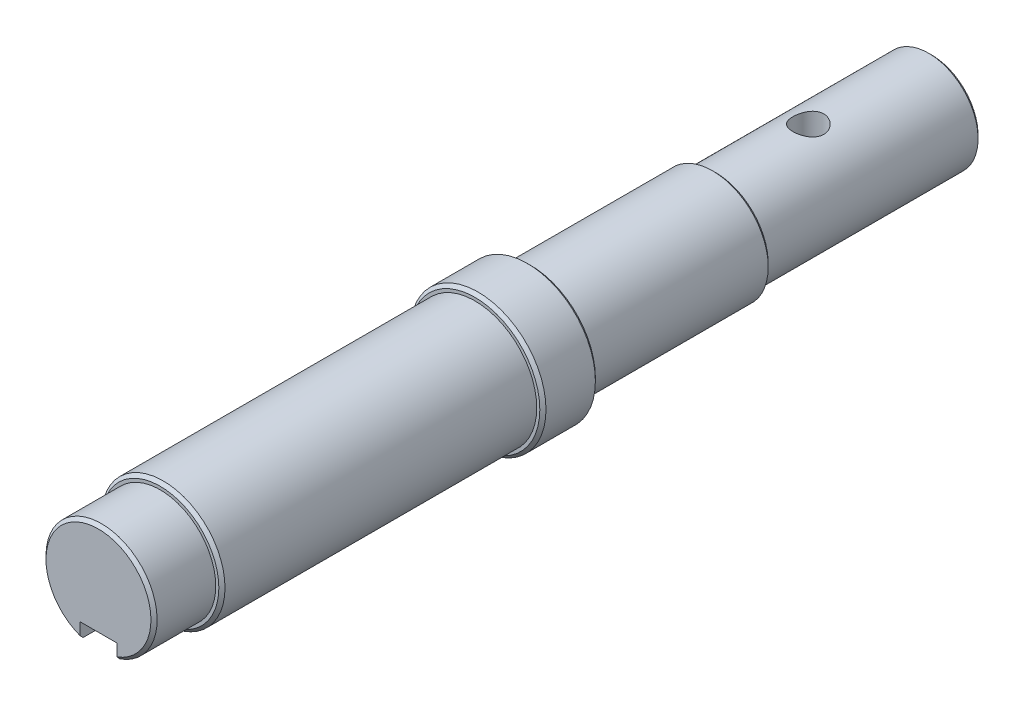
SolidWorks part; units mm, degrees
ref_plane "Front Plane" through (0, 0, 0) normal (0, 0, 1) x (1, 0, 0)
ref_plane "Top Plane" through (0, 0, 0) normal (0, 1, 0) x (1, 0, 0)
ref_plane "Right Plane" through (0, 0, 0) normal (1, 0, 0) x (0, 0, -1)
sketch "Sketch1" plane through (0, 0, 0) normal (0, 0, 1) x (1, 0, 0)
  circle A0 centre (0, 0) radius 11
  dimension "D1" = 22
extrude "Boss-Extrude1" add sketch "Sketch1" along normal mid plane 9
sketch "Sketch2" plane through (0, 0, -4.5) normal (0, 0, -1) x (-1, 0, 0)
  circle A0 centre (0, 0) radius 9
  dimension "D1" = 18
extrude "Boss-Extrude2" add sketch "Sketch2" along normal blind 30
sketch "Sketch3" plane through (0, 0, 4.5) normal (0, 0, 1) x (1, 0, 0)
  circle A0 centre (0, 0) radius 10
  dimension "D1" = 20
extrude "Boss-Extrude3" add sketch "Sketch3" along normal blind 51
sketch "Sketch4" plane through (0, 0, 55.5) normal (0, 0, 1) x (1, 0, 0)
  circle A0 centre (0, 0) radius 9
  dimension "D1" = 18
extrude "Boss-Extrude4" add sketch "Sketch4" along normal blind 10
sketch "Sketch5" plane through (0, 0, 0) normal (0, 1, 0) x (1, 0, 0)
  line L0 (0, -65.5) -> (0, -59.5) construction
  line L1 (-9, -65.5) -> (9, -65.5) construction
  line L2 (-3, -65.5) -> (-3, -59.5)
  line L3 (3, -65.5) -> (3, -59.5)
  line L4 (-9, -55.5) -> (9, -55.5) construction
  arc A0 (-3, -65.5) -> (3, -65.5) centre (0, -65.5) ccw
  arc A1 (3, -59.5) -> (-3, -59.5) centre (0, -59.5) ccw
  point P5 (0, -62.5)
  dimension "D1" = 3
  dimension "D2" = 4
extrude "Cut-Extrude1" cut sketch "Sketch5" against normal blind 15
sketch "Sketch6" plane through (0, 0, 0) normal (0, -1, 0) x (1, 0, 0)
  line L3 (3, 65.5) -> (-3, 65.5)
  line L4 (-3, 65.5) -> (-3, 59.5)
  line L5 (3, 59.5) -> (3, 65.5)
  line L6 (3, 65.5) -> (-3, 65.5)
  line L7 (-3, 65.5) -> (-3, 59.5)
  line L8 (3, 59.5) -> (3, 65.5)
  arc A1 (-3, 59.5) -> (3, 59.5) centre (0, 59.5) ccw
  arc A2 (-3, 59.5) -> (3, 59.5) centre (0, 59.5) ccw
  dimension "D1" = 0
extrude "Boss-Extrude5" add sketch "Sketch6" along normal blind 6
sketch "Sketch7" plane through (0, 0, 0) normal (0, 1, 0) x (1, 0, 0)
  line L0 (0, 10.5) -> (0, 8.5) construction
  line L2 (3, 10.5) -> (3, 8.5)
  line L3 (-3, 10.5) -> (-3, 8.5)
  line L4 (9, 4.5) -> (-9, 4.5) construction
  arc A0 (3, 10.5) -> (-3, 10.5) centre (0, 10.5) ccw
  arc A1 (-3, 8.5) -> (3, 8.5) centre (0, 8.5) ccw
  point P5 (0, 9.5)
  dimension "D1" = 3
  dimension "D2" = 4
  dimension "D3" = 2
extrude "Cut-Extrude2" cut sketch "Sketch7" against normal blind 19
sketch "Sketch8" plane through (0, 0, 0) normal (0, -1, 0) x (1, 0, 0)
  line L4 (3, -10.5) -> (3, -8.5)
  line L5 (-3, -8.5) -> (-3, -10.5)
  line L7 (3, -10.5) -> (3, -8.5)
  line L8 (-3, -8.5) -> (-3, -10.5)
  arc A1 (3, -8.5) -> (-3, -8.5) centre (0, -8.5) ccw
  arc A2 (3, -8.5) -> (-3, -8.5) centre (0, -8.5) ccw
  arc A4 (-3, -10.5) -> (3, -10.5) centre (0, -10.5) ccw
  arc A5 (-3, -10.5) -> (3, -10.5) centre (0, -10.5) ccw
  dimension "D1" = 0
extrude "Boss-Extrude6" add sketch "Sketch8" along normal blind 6
chamfer "Chamfer1" distance 0.5 angle 45 5 edges at (-9, 0, -34.5) (11, 0, -4.5) (11, 0, 4.5) (10, 0, 55.5) (0, 9, 65.5)
sketch "Sketch9" plane through (0, 0, -34.5) normal (0, 0, -1) x (-1, 0, 0)
  circle A0 centre (0, 0) radius 8
  dimension "D1" = 16
extrude "Boss-Extrude7" add sketch "Sketch9" along normal blind 35
cosmetic thread "Cosmetic Thread1" parameters "D1"=20, "D2"=14.376
chamfer "Chamfer2" distance 0.5 angle 45 1 edges at (-8, 0, -69.5)
sketch "Sketch10" plane through (0, 0, 0) normal (0, 1, 0) x (1, 0, 0)
  line L0 (7.5, 69.5) -> (-7.5, 69.5) construction
  line L1 (0, 0) -> (0, 49.5) construction
  circle A0 centre (0, 49.5) radius 2.5
  dimension "D1" = 5
  dimension "D2" = 20
extrude "Cut-Extrude3" cut sketch "Sketch10" against normal mid plane 30
